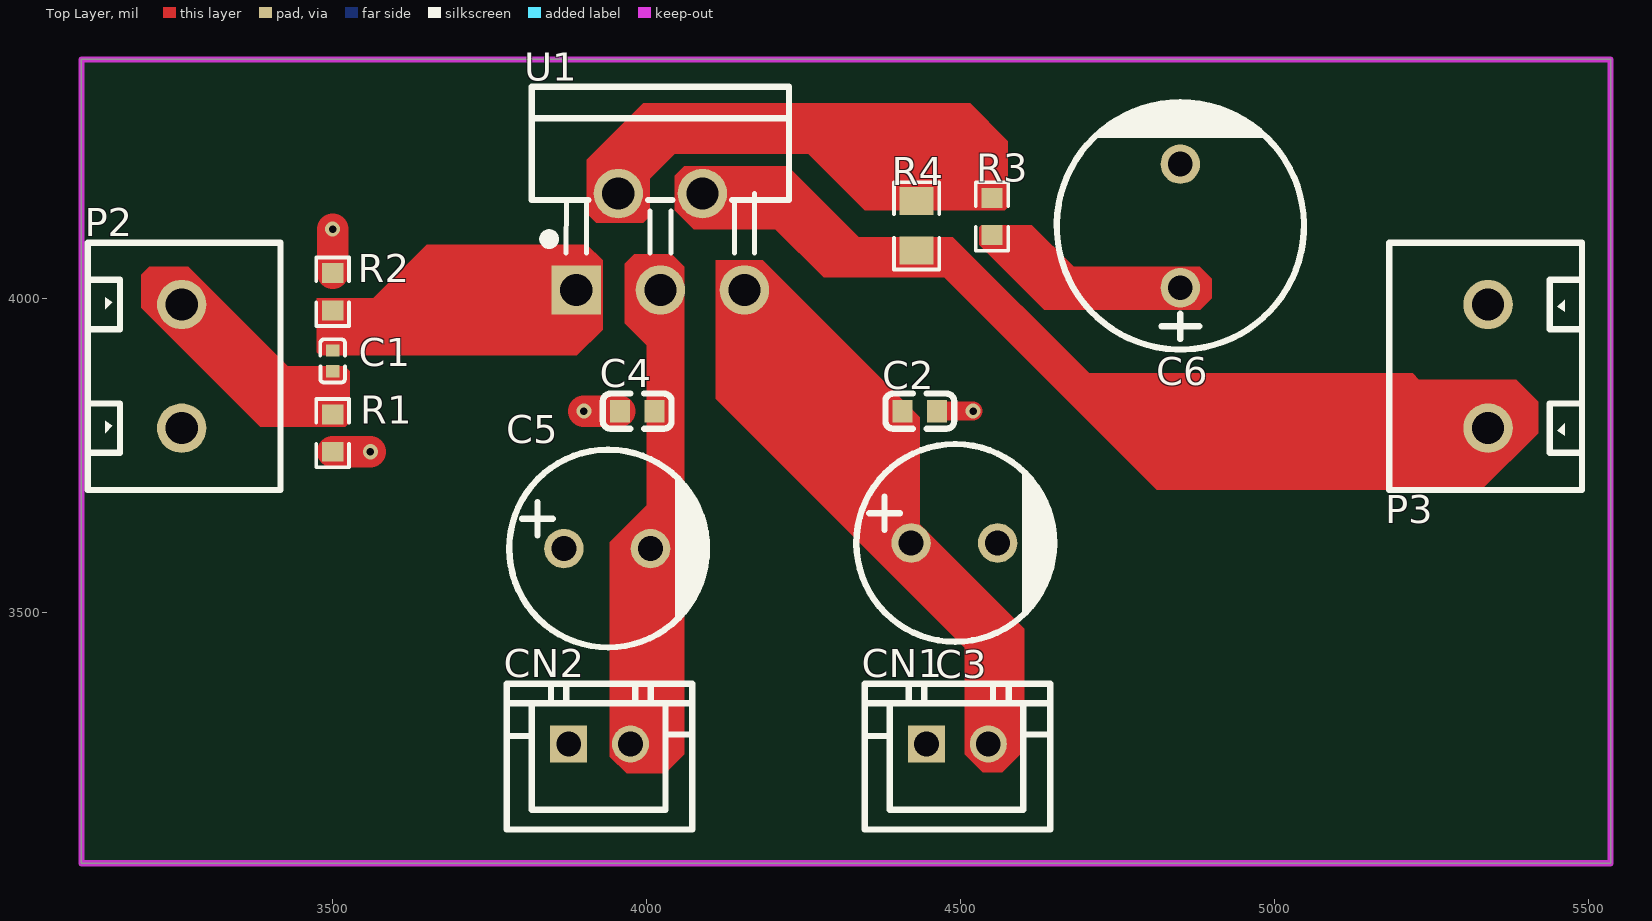
[diagram p0: Top Layer view]
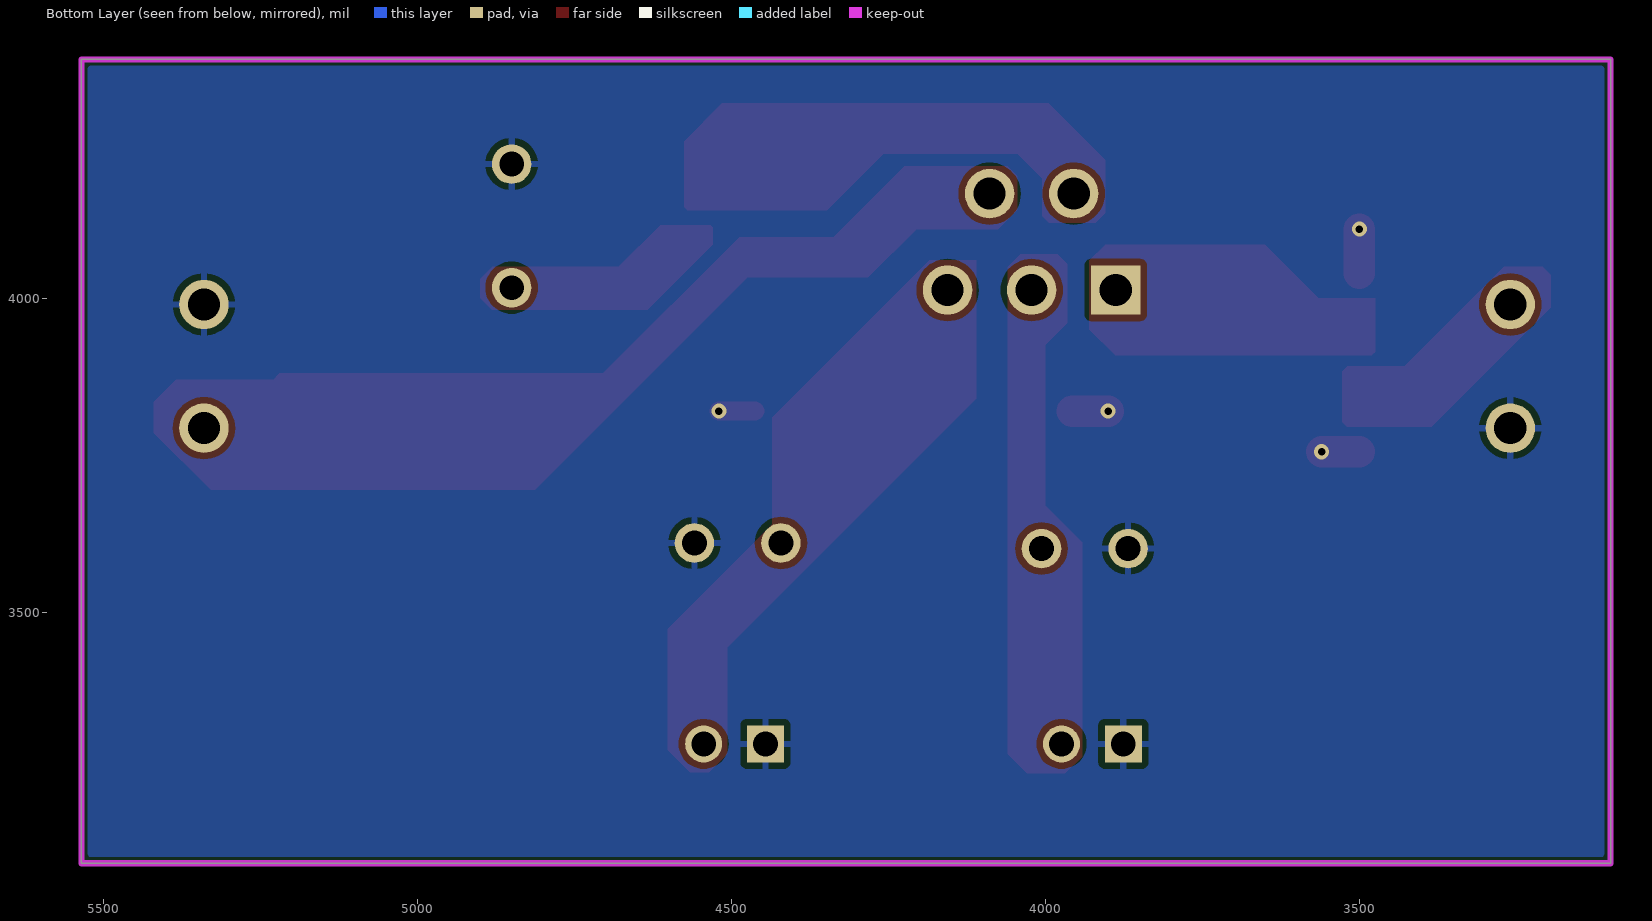
[diagram p1: Bottom Layer view, seen from below]
# Altium PCB MISC82886.pcbdoc
Units mil, origin at the board's own origin, x right, y up, seen from the top; angles counter-clockwise.
Board outline 2435 x 1280 mil, 2 copper layers (Top Layer, Bottom Layer), stack 62.206 mil thick; 15 components, 8 nets, 33 pads, 4 vias.

## Layer stack, top to bottom
Top Solder Mask Layer: solder mask 0.394, Dk 3.3
Top Layer: signal copper 1.379
Dielectric1: surface 59.449, FR4, Dk 4.5
Bottom Layer: signal copper 1.378
Bottom Solder Mask Layer: solder mask 0.394, Dk 3.3

## Board outline
3100,4380 3100,3100 5535,3100 5535,4380

## Design rules (kind name [scope] priority, off if disabled: settings)
BoardOutlineClearance copperThickness2oz_1 [All] p2 off: genericclearance=7.99 ignorepadtopadclearanceinfootprint=FALSE except(0: Arc-SplitContinuation Track-SplitContinuation SMDPad-SplitContinuation THPad-SplitContinuation Via-SplitContinuation Fill-SplitContinuation Region-SplitContinuation Poly-SplitContinuation Text-SplitContinuation Hole-SplitContinuation; 5.98: Arc-CutoutEdge SMDPad-CutoutEdge THPad-CutoutEdge Via-CutoutEdge Fill-CutoutEdge Region-CutoutEdge Text-CutoutEdge; 6.93: Hole-OutlineEdge Hole-CutoutEdge; 10: Poly-OutlineEdge Poly-CutoutEdge; 11.81: Arc-OutlineEdge Track-OutlineEdge SMDPad-OutlineEdge THPad-OutlineEdge Via-OutlineEdge Fill-OutlineEdge Region-OutlineEdge Text-OutlineEdge Track-CutoutEdge)
BoardOutlineClearance copperThickness1oz_1 [All] p4: genericclearance=4.02 ignorepadtopadclearanceinfootprint=FALSE except(0: Arc-SplitContinuation Track-SplitContinuation SMDPad-SplitContinuation THPad-SplitContinuation Via-SplitContinuation Fill-SplitContinuation Region-SplitContinuation Poly-SplitContinuation Text-SplitContinuation Hole-SplitContinuation; 6: SMDPad-CutoutEdge THPad-CutoutEdge Via-CutoutEdge Fill-CutoutEdge Region-CutoutEdge Text-CutoutEdge; 6.93: Hole-OutlineEdge Hole-CutoutEdge; 10: Poly-OutlineEdge Poly-CutoutEdge; 11.8: Arc-OutlineEdge Track-OutlineEdge SMDPad-OutlineEdge THPad-OutlineEdge Via-OutlineEdge Fill-OutlineEdge Region-OutlineEdge Text-OutlineEdge; 11.81: Arc-CutoutEdge Track-CutoutEdge)
Clearance copperThickness2oz [All] p1 off: gap=7.99 ignorepadtopadclearanceinfootprint=FALSE except(5.98: SMDPad-Track SMDPad-SMDPad THPad-Track SMDPad-THPad THPad-THPad Track-Via SMDPad-Via THPad-Via Via-Via Fill-Track Region-Track Fill-SMDPad Region-SMDPad Fill-THPad Region-THPad Fill-Via Region-Via Fill-Fill Fill-Region Region-Region Arc-Track Arc-SMDPad Arc-THPad Arc-Via Fill-Arc Region-Arc Arc-Arc Text-Track SMDPad-Text Text-THPad Text-Via Fill-Text Region-Text Arc-Text Text-Text; 6.93: Hole-Track Hole-SMDPad Hole-THPad Hole-Via Fill-Hole Region-Hole Hole-Arc Hole-Text; 10: Poly-Track Poly-SMDPad Poly-THPad Poly-Via Poly-Fill Poly-Region Poly-Poly Poly-Arc Poly-Text Poly-Hole)
Clearance copperThickness1oz [All] p3: gap=4.02 ignorepadtopadclearanceinfootprint=FALSE except(5.98: SMDPad-Track SMDPad-SMDPad THPad-Track SMDPad-THPad THPad-THPad Track-Via SMDPad-Via THPad-Via Via-Via Fill-Track Region-Track Fill-SMDPad Region-SMDPad Fill-THPad Region-THPad Fill-Via Region-Via Fill-Fill Fill-Region Region-Region; 6: Arc-Track Arc-SMDPad Arc-THPad Arc-Via Fill-Arc Region-Arc Arc-Arc Text-Track SMDPad-Text Text-THPad Text-Via Fill-Text Region-Text Arc-Text Text-Text; 6.93: Hole-Track Hole-SMDPad Hole-THPad Hole-Via Fill-Hole Region-Hole Hole-Arc Hole-Text; 10: Poly-Track Poly-SMDPad Poly-THPad Poly-Via Poly-Fill Poly-Region Poly-Poly Poly-Arc Poly-Text Poly-Hole)
Creepage creepage [All] p1: checkdistance=0 ignoreinternallayers=TRUE applytopolygonpour=TRUE
DiffPairsRouting differentialPair [All] p1: maxlimit=6 minlimit=6 mostfreqgap=6 toplayer_minwidth=5 toplayer_prefwidth=10 toplayer_maxwidth=100 toplayer_mingap=6 toplayer_prefgap=6 toplayer_maxgap=6 bottomlayer_minwidth=5 bottomlayer_prefwidth=10 bottomlayer_maxwidth=100 bottomlayer_mingap=6 bottomlayer_prefgap=6 bottomlayer_maxgap=6 maxuncoupledlength=10
HoleToHoleClearance otherClearance [All] p1: gap=11.81 allowstackedmicrovias=TRUE
Length netLength [All] p1: minlimit=0 maxlimit=0
MatchedLengths netLengthTolerance [All] p1: tolerance=1000
PasteMaskExpansion pasteMaskExpansion [All] p1: expansion=0
PlaneConnect innerPlane [All] p1: planeconnectstyle=Relief reliefexpansion=20 reliefentries=4 reliefconductorwidth=10 reliefairgap=10
PolygonConnect copperRegion [(InNet('GND'))] p1: connectstyle=Relief reliefconductorwidth=10 reliefentries=4 polygonreliefangle="90 Angle" airgapwidth=10 via.connectstyle=Relief via.reliefconductorwidth=10 via.reliefentries=4 via.polygonreliefangle="90 Angle" via.airgapwidth=10
RoutingVias viaSize [All] p1: holewidth=12.01 width=24.02 viastyle="Through Hole" minholewidth=11.81 minwidth=19.68 maxholewidth=248.03 maxwidth=393.7
SolderMaskExpansion solderMaskExpansion [IsVia] p1: expansion=-1000 istentingtop=TRUE
SolderMaskExpansion solderMaskExpansion [All] p2: expansion=2 istentingtop=FALSE
Width copperThickness2oz_2 [All] p1 off: maxlimit=100 minlimit=8 preferedwidth=10
Width copperThickness1oz_2 [All] p2: maxlimit=100 minlimit=5 preferedwidth=10

## Components (designator, comment, footprint, x,y, rotation, side; value= is the part's Value field where it differs from the comment)
C1 "2.2uF" C0402 3500,3900 r90 top
C2 "100nF" C0603 4435,3820 r180 top
C3 "100uF" CAP-TH_BD8.0-P3.50-D0.5-FD 4490,3610 r0 top
C4 "100nF" C0603 3985,3820 r0 top
C5 "100uF" CAP-TH_BD8.0-P3.50-D0.5-FD 3937.22,3601.17 r0 top
C6 "22uF" CAP-TH_BD10.0-P5.00-D0.6-FD 4850,4115 r90 top
CN1 "HX-XH2.54-2PZZ" CONN-TH_2P-P2.50_HX-2.54MM-2P-ZZ-MS 4495,3290 r0 top
CN2 "HX-XH2.54-2PZZ" CONN-TH_2P-P2.50_HX-2.54MM-2P-ZZ-MS 3925,3290 r0 top
P2 "WJ126V-5.0-2P" CONN-TH_WJ126V-5.0-2P 3259.61,3891.34 r0 top
P3 "WJ126V-5.0-2P" CONN-TH_WJ126V-5.0-2P 5340,3891.39 r180 top
R1 "1MΩ" R0603 3500,3785 r90 top
R2 "22kΩ" R0603 3500,4010 r270 top
R3 "1kΩ" R0603 4550,4130 r270 top
R4 "100Ω" R0805 4430,4115 r270 top
U1 "TDA2030A" TO-220B-5_L10.6-W8.7-P1.70-BL 4021.83,4089.66 r0 top

## Footprints (in the part's own frame and the unit in brackets; to place one, negate y for a bottom-side part, rotate by r counter-clockwise, add the part's x,y. Pads: shape width x height; smd on the part's side, far side on the other; paste and mask are expansions set on the pad)
C0402 [mm]
  rect 0.5x0.54 smd: 1(-0.42,0) 2(0.42,0)
  silkscreen extent -0.87,-0.5 0.87,0.5
C0603 [mm]
  rect 0.8x0.9 smd: 1(-0.7,0) 2(0.7,0)
  silkscreen extent -1.39,-0.71 1.39,0.71
CAP-TH_BD8.0-P3.50-D0.5-FD [mm]
  round 1.6 hole 1: 1(-1.75,0) 2(1.75,0)
  silkscreen extent -3.96,-4 4.04,4
CAP-TH_BD10.0-P5.00-D0.6-FD [mm]
  round 1.6 hole 1 paste+0 mask+0.05: 1(-2.5,0) 2(2.5,0)
  silkscreen extent -5,-5 5.08,5
CONN-TH_2P-P2.50_HX-2.54MM-2P-ZZ-MS [mm]
  rect 1.5x1.5 hole 1: 1(-1.25,0)
  round 1.5 hole 1: 2(1.25,0)
  silkscreen extent -3.75,-3.46 3.75,2.44
CONN-TH_WJ126V-5.0-2P [mm]
  round 2 hole 1.3: 1(0,2.501) 2(0,-2.501)
  silkscreen extent -3.8,-5 4,5
R0603 [mil]
  rect 31.75x34.02 smd paste-3937.01 mask+2: 1(-29.66,0) 2(29.66,0)
  silkscreen extent -55,-26 55,26
R0805 [mm]
  rect 1.133x1.377 smd paste-100 mask+0.051: 1(-1,0) 2(1,0)
  silkscreen extent -1.76,-0.92 1.76,0.92
TO-220B-5_L10.6-W8.7-P1.70-BL [mm]
  rect 2x2 hole 1.3: 1(-3.4,-1.95)
  round 2 hole 1.3: 2(-1.7,1.95) 3(0,-1.95) 4(1.7,1.949) 5(3.4,-1.95)
  silkscreen extent -5.21,-0.45 5.21,6.27

## Via types
v1: diameter 24.02, hole 12, Top Layer to Bottom Layer, 4 vias

## Nets (pads, with @x,y where several pads share a name; then routed paths per layer and width w, separated by ;. In a path a pad name is that pad's centre, name@x,y a point inside that pad or via, vN(x,y) a via of type N, cw(c..) or ccw(c..) an arc to the next point about the centre after c; other vN are vias at no path point)
$2N6: R3.1 R4.1 U1.2
$2N12: C1.1 P2.1 R1.2
$2N13: C1.2 R2.2 U1.1
$2N29: P3.1 R4.2 U1.4
$2N35: C6.1 R3.2
GND: C2.1 C3.2 C4.1 C5.1 C6.2 CN1.1 CN2.1 P2.2 P3.2 R1.1 R2.1 | length 245.2
  Top Layer w30: C2.1 v1(4520,3820)
  Top Layer w50: R1.1 v1(3560,3755.34) ; R2.1 v1(3500,4110) ; v1(3900,3820) C4.1
VCC: C2.2 C3.1 CN1.2 U1.5
VEE: C4.2 C5.2 CN2.2 U1.3

## Polygon pours and split planes (outlines as drawn)
GND on Bottom Layer (solid, remove dead copper, pour order 0): 3000,4485 3000,3000 5660,3000 5660,4485

## Keep-outs
Board Outline Layer:
  the board outline again, w10

## Other copper
Top Layer:
  region net $2N12: 3270,4050 3428.64,3891.36 3519.61,3891.36 3527.51,3883.46 3527.51,3802.51 3520,3795 3385,3795 3195,3985 3195,4037.06 3207.94,4050
  region net $2N13: 3475,4000 3565,4000 3650,4085 3905,4085 3930,4060 3930,3950 3888.72,3908.72 3480.33,3908.72 3475,3914.05
  region net VEE: 3980,4070 4040,4070 4060,4050 4060,3273.33 4029.99,3243.32 3968.09,3243.32 3941.49,3269.92 3941.49,3611.49 4000,3670 4000,3925 3965,3960 3965,4055
  region net VCC: 4110,4060 4185,4060 4435,3810 4435,3640 4601.3,3473.7 4601.3,3280.2 4566.1,3245 4535,3245 4506.43,3273.57 4506.43,3443.57 4110,3840
  region net $2N6: 3905,4220 3995,4310 4515,4310 4575,4250 4575,4145 4570,4140 4347.19,4140 4257.19,4230 4045,4230 4005,4190 4005,4130 3995,4120 3920,4120 3905,4135
  region net $2N29: 4045,4195 4060,4210 4225,4210 4337.81,4097.19 4487.81,4097.19 4705,3880 5220,3880 5230,3870 5385,3870 5420,3835 5420,3785 5329.51,3694.51 4812.7,3694.51 4474.18,4033.02 4281.98,4033.02 4205,4110 4075,4110 4045,4140
  region net $2N35: 4529.83,4113.22 4533.03,4116.42 4613.58,4116.42 4680.01,4049.99 4880.99,4049.99 4900,4030.98 4900,3999.54 4881.86,3981.4 4633.43,3981.4 4529.83,4085